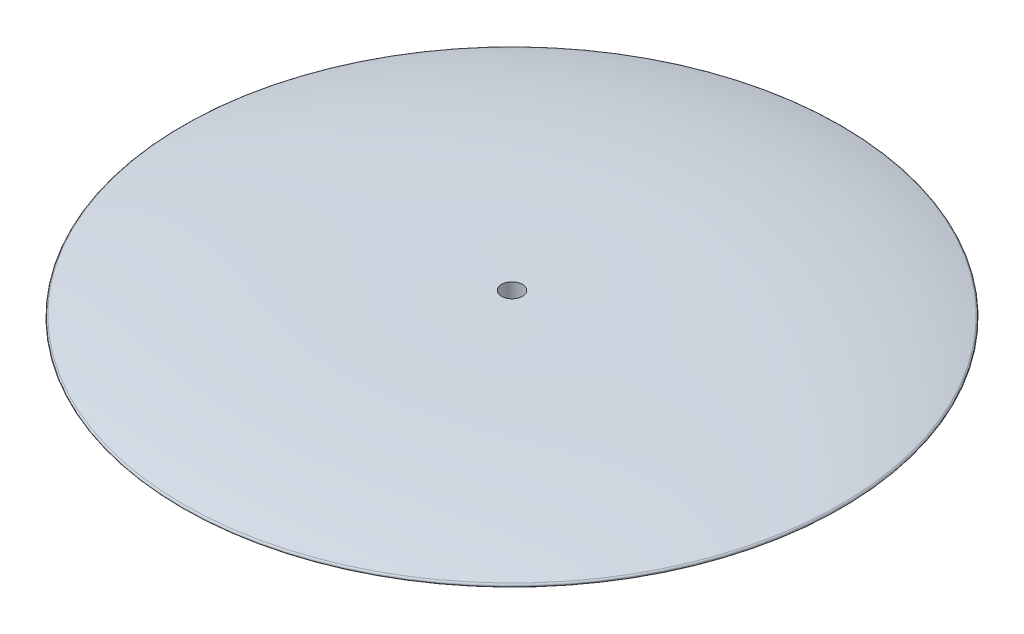
SolidWorks part; units mm, degrees
ref_plane "前视基准面" through (0, 0, 0) normal (0, 0, 1) x (1, 0, 0)
ref_plane "上视基准面" through (0, 0, 0) normal (0, 1, 0) x (1, 0, 0)
ref_plane "右视基准面" through (0, 0, 0) normal (1, 0, 0) x (0, 0, -1)
sketch "草图1" plane through (0, 0, 0) normal (0, 0, 1) x (1, 0, 0)
  line L0 (0, 0) -> (0, -53.5416) construction
  line L1 (0, 0) -> (20.0752, 0) construction
  line L2 (0, -5) -> (25.3471, -5) construction
  line L3 (0, 0) -> (0, -5)
  spline S0 degree 3 poles (-100, -7.8143) (-70.1016, 2.1259) (-22.7748, 0) (0, 0) knots 0 0 0 0 1 1 1 1
  spline S1 degree 3 poles (-100, -7.8143) (-72.0768, -4.0229) (-21.0931, -5) (0, -5) knots 0 0 0 0 1 1 1 1
  dimension "D1" = 100
  dimension "D2" = 5
revolve "旋转1" add sketch "草图1" angle 360 about L0
fillet "圆角1" radius 0.5 1 edges at (0, -7.8143, 100)
sketch "草图2" plane through (0, 0, 0) normal (0, 1, 0) x (1, 0, 0)
  circle A0 centre (0, 0) radius 3
  dimension "D1" = 6
extrude "切除-拉伸1" cut sketch "草图2" against normal mid plane 46
